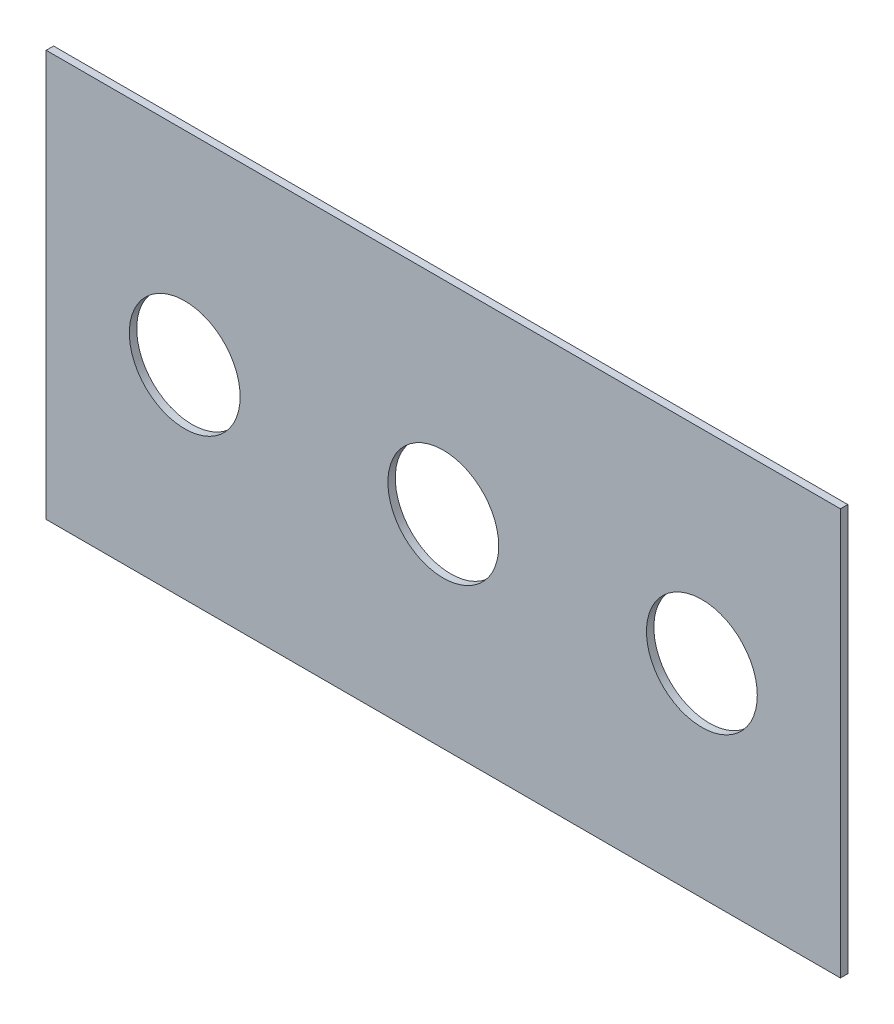
SolidWorks part; units mm, degrees
ref_plane "前视基准面" through (0, 0, 0) normal (0, 0, 1) x (1, 0, 0)
ref_plane "上视基准面" through (0, 0, 0) normal (0, 1, 0) x (1, 0, 0)
ref_plane "右视基准面" through (0, 0, 0) normal (1, 0, 0) x (0, 0, -1)
sketch "草图1" plane through (0, 0, 0) normal (0, 0, 1) x (1, 0, 0)
  line L1 (-21.5, -11) -> (21.5, -11)
  line L2 (-21.5, -11) -> (-21.5, 11)
  line L3 (-21.5, 11) -> (21.5, 11)
  line L4 (21.5, -11) -> (21.5, 11)
  line L5 (-21.5, -11) -> (21.5, 11) construction
  line L6 (-21.5, 11) -> (21.5, -11) construction
  point P0 (0, 0)
  dimension "D1" = 43
  dimension "D2" = 22
extrude "凸台-拉伸1" add sketch "草图1" along normal blind 0.4
sketch "草图2" plane through (0, 0, 0.4) normal (0, 0, 1) x (1, 0, 0)
  circle A0 centre (0, 0) radius 3
  circle A1 centre (-14, 0) radius 3
  circle A2 centre (14, 0) radius 3
  dimension "D1" = 6
  dimension "D2" = 14
  dimension "D3" = 14
extrude "切除-拉伸1" cut sketch "草图2" against normal blind 0.4
